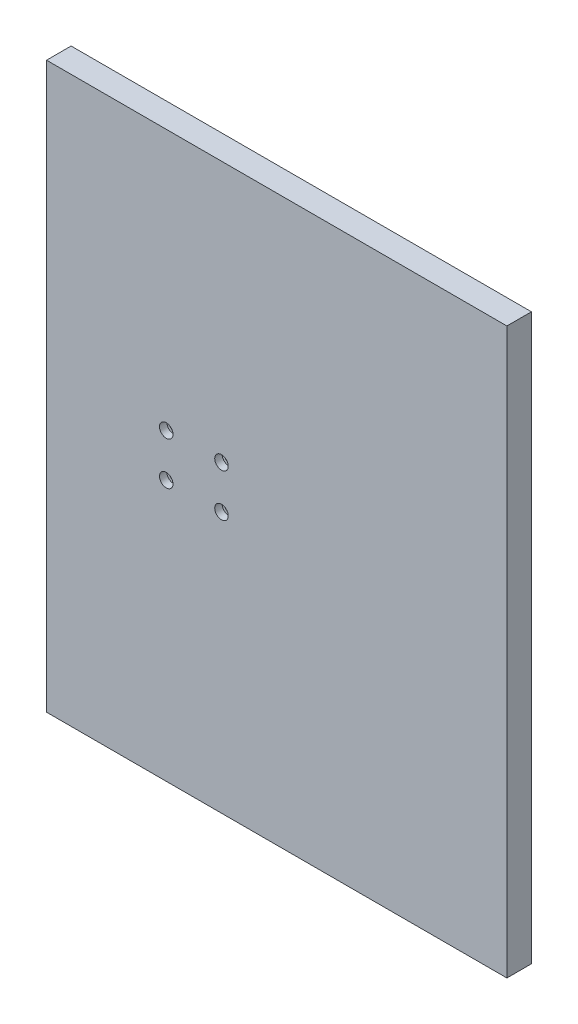
SolidWorks part; units mm, degrees
ref_plane "Front Plane" through (0, 0, 0) normal (0, 0, 1) x (1, 0, 0)
ref_plane "Top Plane" through (0, 0, 0) normal (0, 1, 0) x (1, 0, 0)
ref_plane "Right Plane" through (0, 0, 0) normal (1, 0, 0) x (0, 0, -1)
sketch "Sketch1" plane through (0, 0, 0) normal (0, 0, 1) x (1, 0, 0)
  line L1 (-120, 460) -> (255, 460)
  line L2 (-120, 460) -> (-120, 0)
  line L3 (-120, 0) -> (255, 0)
  line L4 (255, 460) -> (255, 0)
  dimension "D1" = 375
extrude "Boss-Extrude1" add sketch "Sketch1" along normal blind 20 contours L1 L4 L3 L2
hole_wizard "CBORE for M6 Hex Head Bolt1" positions "Sketch2" profile "Sketch3" counterbore size "M6" standard "GB" end condition through all
sketch "Sketch2" plane through (0, 0, 20) normal (0, 0, 1) x (1, 0, 0)
  point P0 (-22.5, 247.5)
  point P3 (22.5, 247.5)
  point P6 (22.5, 212.5)
  point P9 (-22.5, 212.5)
sketch "Sketch3" plane through (-22.5, 247.5, 20) normal (1, 0, 0) x (0, -1, 0)
  line L0 (0, 0) -> (0, 20)
  line L1 (0, 20) -> (3.3, 20)
  line L3 (3.3, 20) -> (3.3, 6)
  line L4 (3.3, 6) -> (5.5, 6)
  line L5 (5.5, 6) -> (5.5, 0)
  line L7 (5.5, 0) -> (0, 0)
  line L11 (0, -6.35) -> (0, 107.95) construction
  dimension "通孔孔直径" = 6.6
  dimension "通孔孔深度" = 20
  dimension "柱形沉头孔直径" = 11
  dimension "柱形沉头孔深度" = 6
